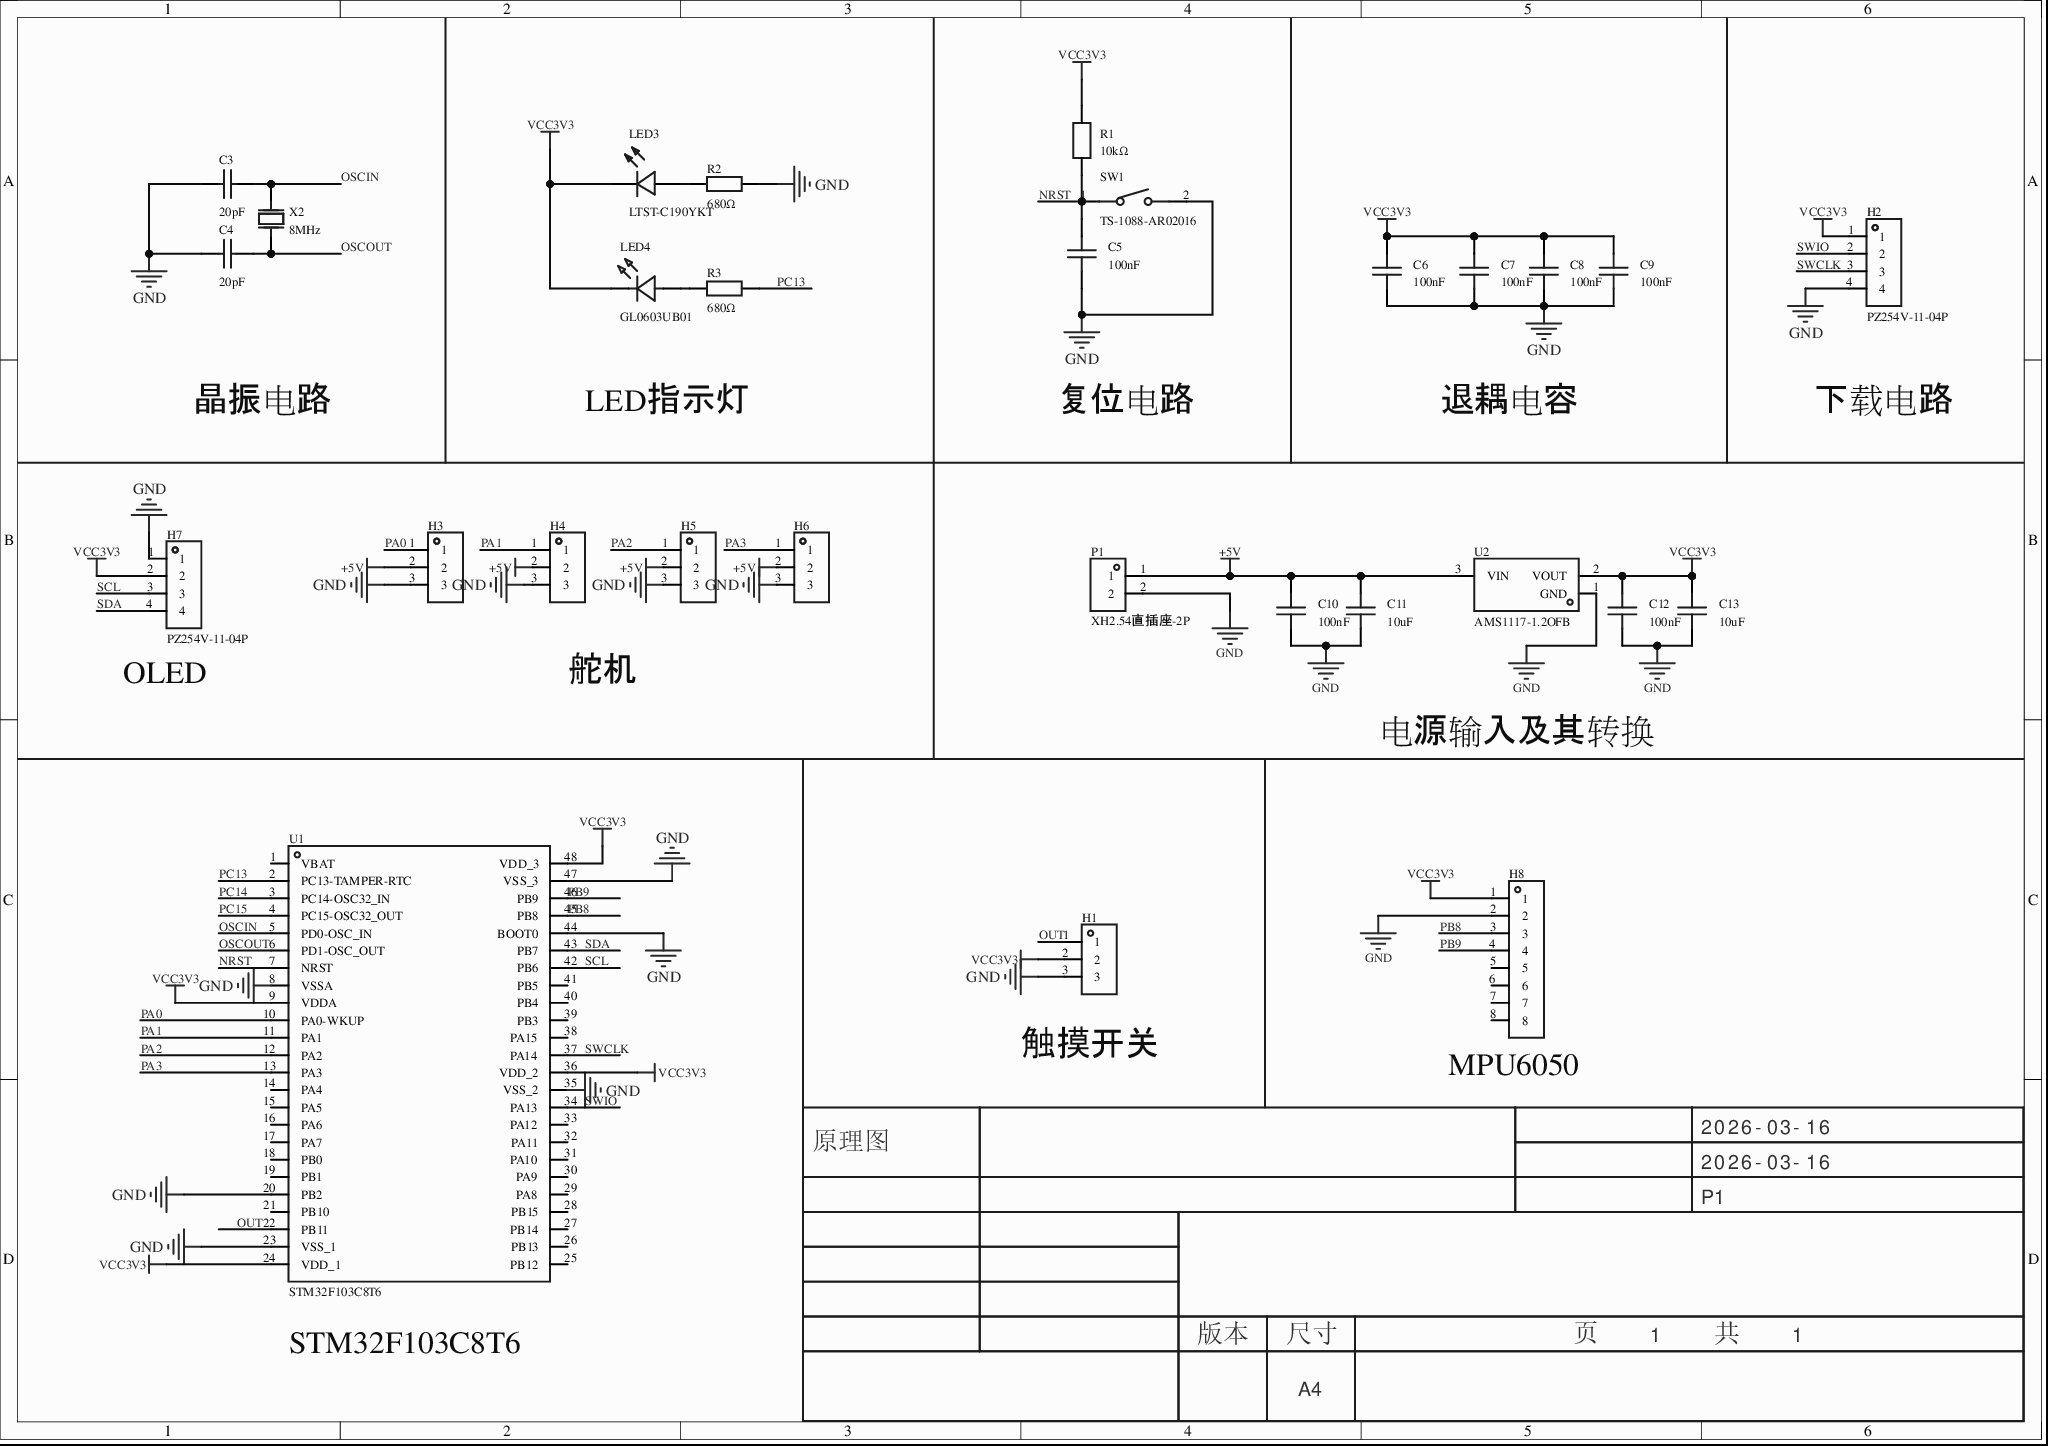
[diagram p0: MISC51388-3.schdoc]
# Altium project MISC51388-2.PrjPcb
1 sheet, 29 parts. Net scope: global (net labels, ports and power ports of the same name join across sheets).
Board file: MISC51388.pcbdoc

## Sheet MISC51388-3.schdoc
size 297 x 209 mm; Version: V1.0; @Project Name: MISC51388; @Page Count: 1; @Update Date: 2026-03-16; @Create Date: 2026-03-16; @Schematic Name: MISC51388; @Page No: 1; @Board Name: MISC51388; @Create Time: 15:50:55; @Update Time: 15:50:55; Size: A4

### Parts
C3  20pF  [C0603]
C4  20pF  [C0603]
C5  100nF  [C0603]
C6  100nF  [C0603]
C7  100nF  [C0603]
C8  100nF  [C0603]
C9  100nF  [C0603]
C10  100nF  [C0603]
C11  10uF  [C0603]
C12  100nF  [C0603]
C13  10uF  [C0603]
H1  (no value)  [HDR-TH_3P-P2.54-V-F]
H2  PZ254V-11-04P  [HDR-TH_4P-P2.54-V-M]
H3  (no value)  [HDR-TH_3P-P2.54-V-M]
H4  (no value)  [HDR-TH_3P-P2.54-V-M]
H5  (no value)  [HDR-TH_3P-P2.54-V-M]
H6  (no value)  [HDR-TH_3P-P2.54-V-M]
H7  PZ254V-11-04P  [HDR-TH_4P-P2.54-V-M]
H8  (no value)  [HDR-TH_8P-P2.54-V-F-1]
LED3  LTST-C190YKT  [LED0603-RD]
LED4  GL0603UB01  [LED0603-RD_BLUE]
P1  XH2.54直插座-2P  [CONN-TH_XH2.54-2P]
R1  10kΩ  [R0603]
R2  680Ω  [R0603]
R3  680Ω  [R0603]
SW1  TS-1088-AR02016  [SW-SMD_L3.9-W3.0-P4.45]
U1  STM32F103C8T6  [LQFP-48_L7.0-W7.0-P0.50-LS9.0-BL]
U2  AMS1117-1.2OFB  [SOT-89-3_L4.5-W2.4-P1.50-LS4.0-BR]
X2  8MHz  [CRYSTAL-SMD_L5.0-W3.2]

### Nets
+5V: C10.2 C11.2 H3.2 H4.2 H5.2 H6.2 P1.1 U2.3(VIN)
GND: C3.1 C4.1 C5.1 C6.1 C7.1 C8.1 C9.1 C10.1 C11.1 C12.1 C13.1 H1.3 H2.4 H3.3 H4.3 H5.3 H6.3 H7.1 H8.2 P1.2 R2.2 SW1.2 U1.8(VSSA) U1.20(PB2) U1.23(VSS_1) U1.35(VSS_2) U1.44(BOOT0) U1.47(VSS_3) U2.1(GND)
VCC3V3: C6.2 C7.2 C8.2 C9.2 C12.2 C13.2 H1.2 H2.1 H7.2 H8.1 LED3.1(-) LED4.1(K) R1.2 U1.9(VDDA) U1.24(VDD_1) U1.36(VDD_2) U1.48(VDD_3) U2.2(VOUT)
NRST: C5.2 R1.1 SW1.1 U1.7(NRST)
OSCIN: C3.2 U1.5(PD0-OSC_IN) X2.2(OSC2)
OSCOUT: C4.2 U1.6(PD1-OSC_OUT) X2.1(OSC1)
OUT: H1.1 U1.22(PB11)
PA0: H3.1 U1.10(PA0-WKUP)
PA1: H4.1 U1.11(PA1)
PA2: H5.1 U1.12(PA2)
PA3: H6.1 U1.13(PA3)
PB8: H8.3 U1.45(PB8)
PB9: H8.4 U1.46(PB9)
PC13: R3.2 U1.2(PC13-TAMPER-RTC)
PC14: U1.3(PC14-OSC32_IN)
PC15: U1.4(PC15-OSC32_OUT)
SCL: H7.3 U1.42(PB6)
SDA: H7.4 U1.43(PB7)
SWCLK: H2.3 U1.37(PA14)
SWIO: H2.2 U1.34(PA13)
NetLED3_2: LED3.2(+) R2.1
NetLED4_2: LED4.2(A) R3.1

Not connected (* = marked no-connect by the designer): H8 5* 6* 7* 8*; U1 1(VBAT)* 14(PA4)* 15(PA5)* 16(PA6)* 17(PA7)* 18(PB0)* 19(PB1)* 21(PB10)* 25(PB12)* 26(PB13)* 27(PB14)* 28(PB15)* 29(PA8)* 30(PA9)* 31(PA10)* 32(PA11)* 33(PA12)* 38(PA15)* 39(PB3)* 40(PB4)* 41(PB5)*

### Notes on the sheet
- 晶振电路
- LED指示灯
- 复位电路
- 退耦电容
- 下载电路
- (near H7) OLED
- 舵机
- 电源输入及其转换
- (near H1) 触摸开关
- (near H8) MPU6050
- (near U1) STM32F103C8T6
- 2026-03-16
- 原理图
- P1
- 版本
- 尺寸
- A4
- 页    1    共    1

### Library data of the parts
C3 C4 = CL10C200JB8NNNC: 容值:20pF;精度:±5%;额定电压:50V;温度系数:C0G;; Manufacturer: SAMSUNG(三星); AddInBom: yes; ModelId: ac125912035d415993ca9572d50418b1; ModelName: C0603_L1.6-W0.8-H0.8; ModelTransform: 62.992,31.496,0,0,0,0,0,0,0; Tolerance: ±5%; Voltage Rating: 50V; Temperature Coefficient: C0G; Symbol: CL10C200JB8NNNC; Device: CL10C200JB8NNNC; LCSC Part Name: 20pF ±5% 50V; SupplierPart: C1648; ManufacturerPart: CL10C200JB8NNNC; Supplier Footprint: 0603; JLCPCB Part Class: 基础库; Datasheet: https://item.szlcsc.com/datasheet/CL10C200JB8NNNC/2000.html; Supplier: LCSC; ConvertToPcb: yes; FootprintName: C0603; Value: 20pF
C5-C9 = CGA0603X7R104K500JT: 容值:100nF;精度:±10%;额定电压:50V;温度系数:X7R;; Manufacturer: HRE(芯声); AddInBom: yes; ModelId: ac125912035d415993ca9572d50418b1; ModelName: C0603_L1.6-W0.8-H0.8; ModelTransform: 62.992,31.496,0,0,0,0,0,0,0; Tolerance: ±10%; Voltage Rating: 50V; Temperature Coefficient: X7R; Symbol: CGA0603X7R104K500JT; Device: CGA0603X7R104K500JT; LCSC Part Name: 100nF ±10% 50V; SupplierPart: C6119867; ManufacturerPart: CGA0603X7R104K500JT; Supplier Footprint: 0603; JLCPCB Part Class: 扩展库; Datasheet: https://item.szlcsc.com/datasheet/CGA0603X7R104K500JT/7062573.html; Supplier: LCSC; ConvertToPcb: yes; FootprintName: C0603; Value: 100nF
C10-C13 = CAP_0603: Symbol: Capacitance; ConvertToPcb: yes; ModelId: ac125912035d415993ca9572d50418b10819f05c4eef4c71ace90d822a990e87; ModelName: C0603_L1.6-W0.8-H0.8; ModelTransform: 62.992,31.496,0,0,0,0,0,0,0; Device: CAP_0603; AddInBom: yes; Supplier Footprint: 0603; FootprintName: C0603
  C10 C12: Value: 100nF
  C11 C13: Value: 10uF
H1 = HDR-F_2.54_1x3P: Symbol: PM254V-11-03-H85; ConvertToPcb: yes; ModelId: f3b3cc5aae9641bf9e56fc160cef875b0819f05c4eef4c71ace90d822a990e87; ModelName: HDR2.54-F-LI-1X3P; ModelTransform: 299.9994,100,0,0,0,0,0,0,-118.11; Device: HDR-F_2.54_1x3P; AddInBom: yes; SupplierPart: C541850; Supplier Footprint: 插件; FootprintName: HDR-TH_3P-P2.54-V-F
H2 H7 = PZ254V-11-04P: 插针结构:1x4P;间距:2.54mm;行距:-;圆针/方针:方针;安装方式:直插;排数:单排;总PIN位数:4P;额定电流:3A;额定电压:250V;配合针长度:6mm;塑高:2.5mm;端接针长度:3mm;触头材质:-;工作温度:-40℃~+105℃;颜色:黑色;; Manufacturer: XFCN(兴飞); Symbol: PZ254V-11-04P_C2691448; AddInBom: yes; ModelId: 112f4d05e8d64e99ab9a333894bea4f9; ModelName: HDR-TH_4P-P2.54-M-LI-1X4P; ModelTransform: 399.999,104.7242,0,0,0,0,0,0,-118.11; Pin Structure: 1x4P; Pitch: 2.54mm; Circluar Pins/Square Pins: 方针; Current Rating: 3A; Voltage Rating (Max): 250V; Device: PZ254V-11-04P; LCSC Part Name: 1x4P 间距:2.54mm 方针 直插; SupplierPart: C2691448; ManufacturerPart: PZ254V-11-04P; Supplier Footprint: 插件,P=2.54mm; JLCPCB Part Class: Extended Part; Datasheet: https://item.szlcsc.com/datasheet/PZ254V-11-04P/2801085.html; Supplier: LCSC; ConvertToPcb: yes; FootprintName: HDR-TH_4P-P2.54-V-M; Row Spacing: -; Mounting Type: 直插; Number of Rows: 单排; Number of Pins: 4P; Length of Mating Pin: 6mm; Insulation Height: 2.5mm; Length of End Connection Pin: 3mm; Contact Material: -; Operating Temperature: -40℃~+105℃; Color: 黑色
H3-H6 = HDR-M_2.54_1x3P: AddInBom: yes; ModelId: bb473b6d38ff42a99216a4fcdbdcc4cb0819f05c4eef4c71ace90d822a990e87; ModelName: HDR-TH_3P-P2.54-M-LI-1X3P; ModelTransform: 300.03877,100,0,0,0,0,0,0,-118.11; Symbol: HDR-M_2.54_1x3P; Device: HDR-M_2.54_1x3P; ConvertToPcb: yes; FootprintName: HDR-TH_3P-P2.54-V-M; SupplierPart: C2937625; Supplier Footprint: 插件
H8 = HDR-F_2.54_1x8P: Symbol: Header-Female-2.54_1x8; AddInBom: yes; ModelId: 0f7e4d9227ef4fa08d5469c22cc70cdb0819f05c4eef4c71ace90d822a990e87; ModelName: HDR-F-2.54_1x8; ModelTransform: 799.99844,100,0,0,0,0,0,0,-118.11; Device: HDR-F_2.54_1x8P; ConvertToPcb: yes; FootprintName: HDR-TH_8P-P2.54-V-F-1; SupplierPart: C27438; Supplier Footprint: 插件
LED3 = LTST-C190YKT: 发光颜色:黄色;正向压降(Vf):2.1V;功率:60mW;正向电流:20mA;波长:588nm;二极管配置:-;透镜颜色:无色透明透镜;色温:-;发光强度:6mcd;发光角度:130°;载带方式:-;工作温度:-55℃~+85℃;; Manufacturer: LITEON(光宝); AddInBom: yes; ModelId: 1f0d29a91be547639d425604e9b96ebb; ModelTransform: 63.7794,32.283,0,0,0,0,0,0,0; Illumination Color: 黄色; Voltage - Forward(Vf): 2.1V; Power(Watts): 60mW; Forward Current: 20mA; Wavelength - Dominant: 588nm; Peak Wavelength: 585nm; Lens Color: 无色透明透镜; Luminous Intensity: 6mcd; Viewing Angle: 130°; Symbol: LTST-C190YKT; Device: LTST-C190YKT; LCSC Part Name: 黄灯; SupplierPart: C125097; ManufacturerPart: LTST-C190YKT; Supplier Footprint: 0603; JLCPCB Part Class: 扩展库; Datasheet: https://item.szlcsc.com/datasheet/LTST-C190YKT/136373.html; Supplier: LCSC; ConvertToPcb: yes; FootprintName: LED0603-RD; ModelName: LED0603-RD; Diode Configuration: -; Color Temperature: -; Mounting Style: -; Operating Temperature: -55℃~+85℃
LED4 = GL0603UB01: 发光颜色:蓝色;正向压降(Vf):2.9V;正向电流:20mA;波长:460nm~469nm;二极管配置:独立二极管;透镜颜色:无色透明透镜;发光强度:72mcd;发光角度:120°;载带方式:正贴;工作温度:-40℃~+85℃;; Manufacturer: Guiguang light(桂光光电); AddInBom: yes; ModelId: 9a6c0bc6a1b149eb93d2e332f32d5db3; ModelTransform: 63.7794,31.496,0,0,0,0,0,0.002,0; Illumination Color: 蓝色; Voltage - Forward(Vf): 2.9V; Forward Current: 20mA; Diode Configuration: 独立二极管; Lens Color: 无色透明透镜; Luminous Intensity: 72mcd; Viewing Angle: 120°; Symbol: GL0603UB01; Device: GL0603UB01; LCSC Part Name: 0603 蓝灯 高亮; SupplierPart: C51933294; ManufacturerPart: GL0603UB01; Supplier Footprint: 0603; JLCPCB Part Class: 扩展库; Datasheet: https://item.szlcsc.com/datasheet/GL0603UB01/54645990.html; Supplier: LCSC; ConvertToPcb: yes; FootprintName: LED0603-RD_BLUE; ModelName: LED0603-RD_BLUE; Wavelength - Dominant: 460nm~469nm; Mounting Style: 正贴; Operating Temperature: -40℃~+85℃
P1 = XH2.54直插座-2P: AddInBom: yes; ModelId: c3cc11bd8b8748c1ae6bc231aac3a1ff0819f05c4eef4c71ace90d822a990e87; ModelTransform: 296.889,230.315,0,0,0,0,0,26.653,-137.795; Symbol: XH2.54直插座-2P; Device: XH2.54直插座-2P; LCSC Part Name: XH2.54直插座-2P; SupplierPart: C9900016957; ManufacturerPart: XH2.54直插座-2P; Supplier Footprint: XH2.54-2; JLCPCB Part Class: Extended Part; Supplier: LCSC; ConvertToPcb: yes; FootprintName: CONN-TH_XH2.54-2P; ModelName: CONN-TH_XH2.54-2P
R1 = AST0310KF: 阻值:10kΩ;精度:±1%;功率:100mW;工作电压:75V;温度系数:±100ppm/℃;; Manufacturer: HKR(香港电阻); AddInBom: yes; ModelId: fc143cca1e79419f9cd78b61e9279f08; ModelTransform: 31.8897,63.7794,0,90,0,0,0,0,0; Tolerance: ±1%; Power(Watts): 100mW; Voltage-Supply(Max): 75V; Symbol: AST0310KF; Device: AST0310KF; LCSC Part Name: 10K ±1%; SupplierPart: C49330116; ManufacturerPart: AST0310KF; Supplier Footprint: 0603; JLCPCB Part Class: 扩展库; Datasheet: https://item.szlcsc.com/datasheet/AST0310KF/51811758.html; Supplier: LCSC; ConvertToPcb: yes; FootprintName: R0603; ModelName: R0603; Value: 10kΩ; Temperature Coefficient: ±100ppm/℃; Operating Temperature: -55℃~+155℃
R2 R3 = 0603WAF6800T5E: 电阻类型:厚膜电阻;阻值:680Ω;精度:±1%;功率:100mW;最大工作电压:75V;温度系数:±100ppm/℃;; Manufacturer: UNI-ROYAL(厚声); AddInBom: yes; ModelId: fc143cca1e79419f9cd78b61e9279f08; ModelTransform: 31.8897,63.7794,0,90,0,0,0,0,0; Tolerance: ±1%; Power(Watts): 100mW; Overload Voltage (Max): 75V; Symbol: 0603WAF6800T5E; Device: 0603WAF6800T5E; LCSC Part Name: 680Ω ±1% 100mW 厚膜电阻; SupplierPart: C23228; ManufacturerPart: 0603WAF6800T5E; Supplier Footprint: 0603; JLCPCB Part Class: 基础库; Datasheet: https://atta.szlcsc.com/upload/public/pdf/source/20200306/C422600_1E6D84923E4A46A82E41ADD87F860B5C.pdf; Supplier: LCSC; ConvertToPcb: yes; FootprintName: R0603; ModelName: R0603; Type: 厚膜电阻; Value: 680Ω; Temperature Coefficient: ±100ppm/℃; Operating Temperature Range: -55℃~+155℃
SW1 = TS-1088-AR02016: 电路结构:单刀单掷;按钮形状:圆形按钮;作用力:1.6N;安装方式:立贴;开关长度:4mm;开关宽度:3mm;开关高度:2mm;带支架:不带支架;触点电流:50mA;额定电压:12V;工作寿命:10万次;; Manufacturer: XUNPU(讯普); AddInBom: yes; ModelId: b26698b69f274ffabef8a26c7d0e5dd1; ModelName: SW-SMD_L3.9-W2.9-H2.0-LS4.8; ModelTransform: 188.976,114.174,0,0,0,0,0,0,0; Circuit: 单刀单掷; Actuator Style: 圆形按钮; Operating Force: 1.6N; Switch Height: 2mm; with Bracket: 不带支架; Contact Current: 50mA; Voltage Rating: 12V; Actuator/Cap Color: 黑色; Life: 10万次; Symbol: TS-1088-AR02016; Device: TS-1088-AR02016; LCSC Part Name: 4*3*2mm 立贴 轻触开关; SupplierPart: C720477; ManufacturerPart: TS-1088-AR02016; Supplier Footprint: SMD,4x3mm; JLCPCB Part Class: 基础库; Datasheet: https://item.szlcsc.com/datasheet/TS-1088-AR02016/763484.html; Supplier: LCSC; ConvertToPcb: yes; FootprintName: SW-SMD_L3.9-W3.0-P4.45; Mounting Type: 立贴; Length: 4mm; Width: 3mm; Termination Style: SMD接片; Operating Temperature: -30℃~+80℃
U1 = STM32F103C8T6: CPU内核:ARM-M3;CPU最大主频:72MHz;应用领域:-;; Manufacturer: ST(意法半导体); AddInBom: yes; ModelId: 093be70396ff421eb2cdb946d5311efc; ModelName: LQFP-48_L7.0-W7.0-H1.4-LS9.0-P0.50; ModelTransform: 354.331,354.331,0,0,0,0,0,0,0; CPU Core: ARM-M3; CPU Maximum Speed: 72MHz; Program Storage Size: 64KB; Program Memory Type: FLASH; Number of I/O: 37; ADC (Bit): 12bit; Voltage - Supply: 2V~3.6V; Symbol: STM32F103C8T6; Device: STM32F103C8T6; LCSC Part Name: 主流增强型ARM Cortex-M3 MCU，具有64 KB Flash、72 MHz CPU、电机控制、USB和CAN; SupplierPart: C8734; ManufacturerPart: STM32F103C8T6; Supplier Footprint: LQFP-48(7x7); JLCPCB Part Class: 扩展库; Datasheet: https://item.szlcsc.com/datasheet/STM32F103C8T6/9243.html; Supplier: LCSC; ConvertToPcb: yes; FootprintName: LQFP-48_L7.0-W7.0-P0.50-LS9.0-BL; Applications: -
U2 = AMS1117-1.2OFB: 输出类型:固定;工作电压:15V;输出电压:1.2V;输出电流:1A;电源纹波抑制比(PSRR):-;输出极性:正极;; Manufacturer: GMIC(绿微); AddInBom: yes; ModelId: dde435042bae4b9691e74da94cf9d9f30819f05c4eef4c71ace90d822a990e87; ModelTransform: 177.165,161.417,0,90,0,0,-2.323,0,0; Output Type: 固定; Voltage - Supply: 15V; Output Voltage: 1.2V; Output Current: 1A; standby current: 4mA; Output Configuration: 正极; Number of Outputs: 1; Symbol: AMS1117-1.2OFB; Device: AMS1117-1.2OFB; LCSC Part Name: AMS1117-1.2OFB; SupplierPart: C50313798; ManufacturerPart: AMS1117-1.2OFB; Supplier Footprint: SOT-89; JLCPCB Part Class: Extended Part; Datasheet: https://item.szlcsc.com/datasheet/AMS1117-1.2OFB/52904754.html; Supplier: LCSC; ConvertToPcb: yes; FootprintName: SOT-89-3_L4.5-W2.4-P1.50-LS4.0-BR; ModelName: SOT-89-3_L4.5-W2.4-P1.50-LS4.0-BR; Power Supply Rejection Ratio (PSRR): -; Voltage Dropout: -; Noise: -; Features: 短路保护；过压保护; Operating Temperature: -40℃~+125℃@(Ta)
X2 = X50328MSB2GI: 晶振类型:贴片晶振;频率:8MHz;常温频差:±10ppm;负载电容:20pF;频率稳定度:±20ppm;; Manufacturer: YXC(扬兴晶振); AddInBom: yes; ModelId: d7c39c66443246ff83c2003c1e1eb6f1; ModelTransform: 196.85,125.984,0,0,0,0,0,0,0; Normal temperature Frequency Tolerance: ±10ppm; Load Capacitance: 20pF; Frequency Stability: ±20ppm; Symbol: X50328MSB2GI; Device: X50328MSB2GI; LCSC Part Name: YSX530GA 8MHZ 2P 5032 20PF ±10PPM -40~85℃ (±20PPM); SupplierPart: C115962; ManufacturerPart: X50328MSB2GI; Supplier Footprint: SMD5032-2P; JLCPCB Part Class: 基础库; Datasheet: https://item.szlcsc.com/datasheet/X50328MSB2GI/117214.html; Supplier: LCSC; ConvertToPcb: yes; FootprintName: CRYSTAL-SMD_L5.0-W3.2; ModelName: CRYSTAL-SMD_L5.0-W3.2; Type: 贴片晶振; Value: 8MHz; Operating Temperature: -40℃~+85℃